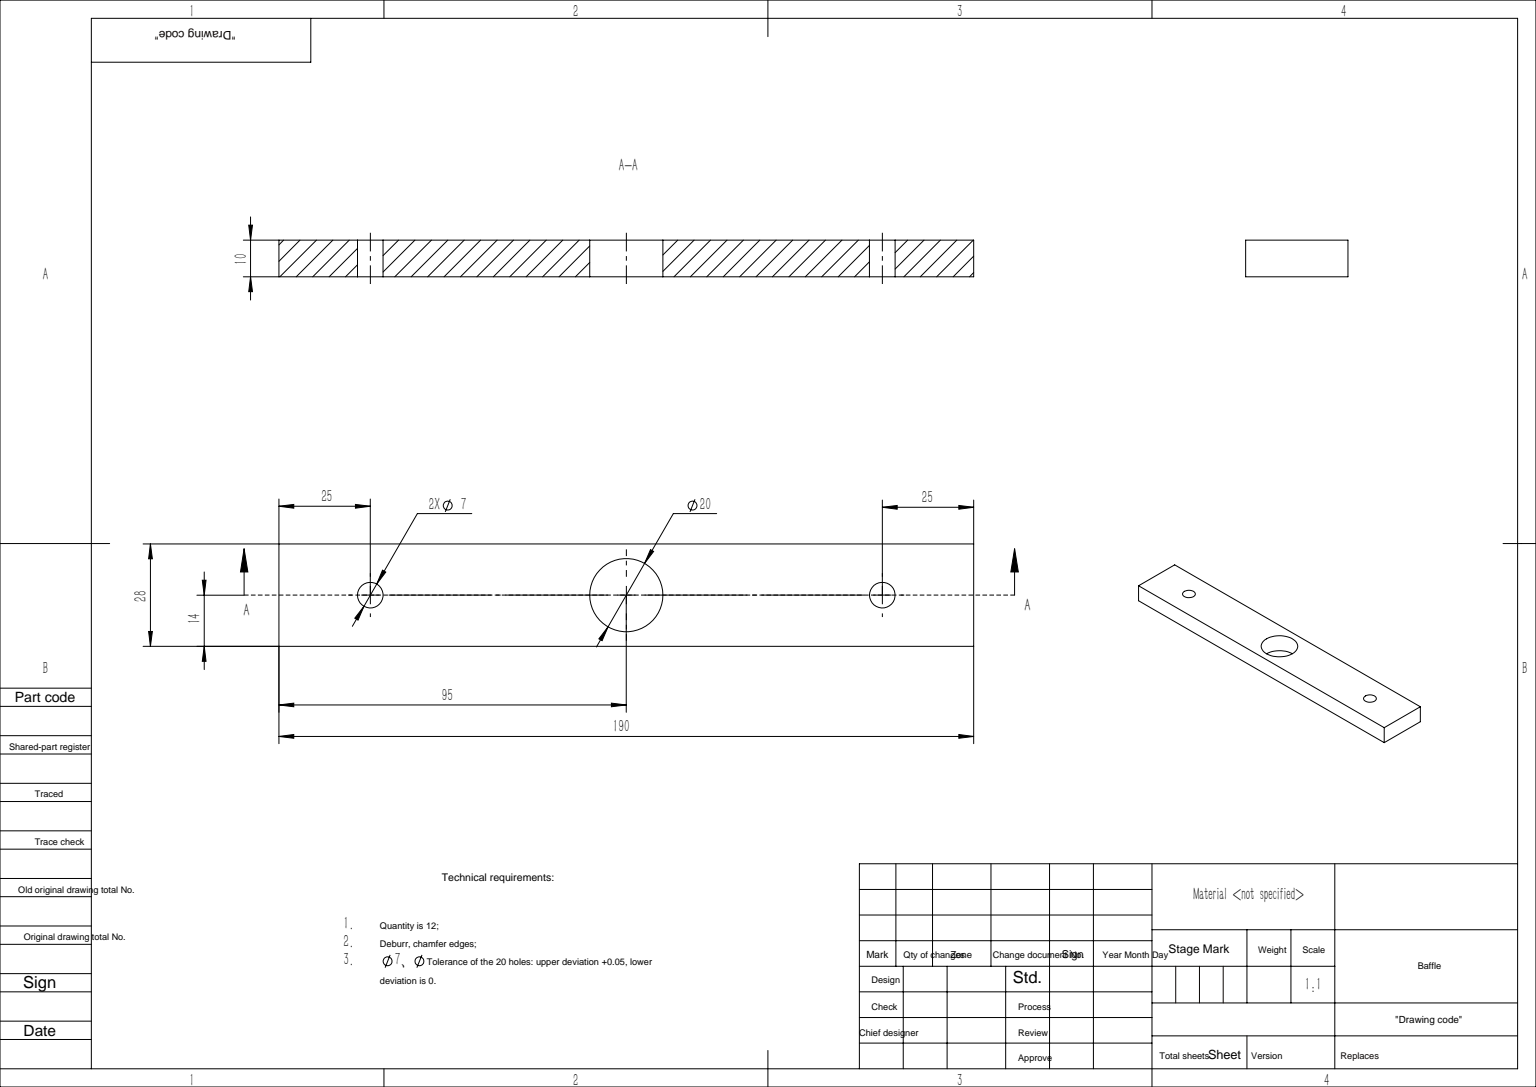
from build123d import *

# Parameters (mm, degrees)
SKETCH_1_W          = 190
SKETCH_1_H          = 28
EXTRUDE_1_DEPTH     = 10
SKETCH_2_R          = 3.5
SKETCH_2_R_2        = 10
CUT_EXTRUDE_1_DEPTH = 846.854305824


with BuildPart() as part:
    # 草图1 → 凸台-拉伸1 (new body)
    with BuildSketch(Plane(origin=(0, 1805.000303929, 0), x_dir=(1, 0, 0), z_dir=(0, 1, 0))):
        with Locations((602.085724054, 465)):
            Rectangle(SKETCH_1_W, SKETCH_1_H)
    extrude(amount=EXTRUDE_1_DEPTH)

    # 草图2 → 切除-拉伸1 (cut, through all)
    with BuildSketch(Plane(origin=(0, 1815.000303929, 0), x_dir=(1, 0, 0), z_dir=(0, 1, 0))):
        with Locations(Location((532.085724054, 465, 0), (0, 0, 180))):
            Circle(SKETCH_2_R)
        with Locations(Location((672.085724054, 465, 0), (0, 0, 180))):
            Circle(SKETCH_2_R)
        with Locations(Location((602.085724054, 465, 0), (0, 0, 180))):
            Circle(SKETCH_2_R_2)
    extrude(amount=-CUT_EXTRUDE_1_DEPTH, mode=Mode.SUBTRACT)


solid = part.part
